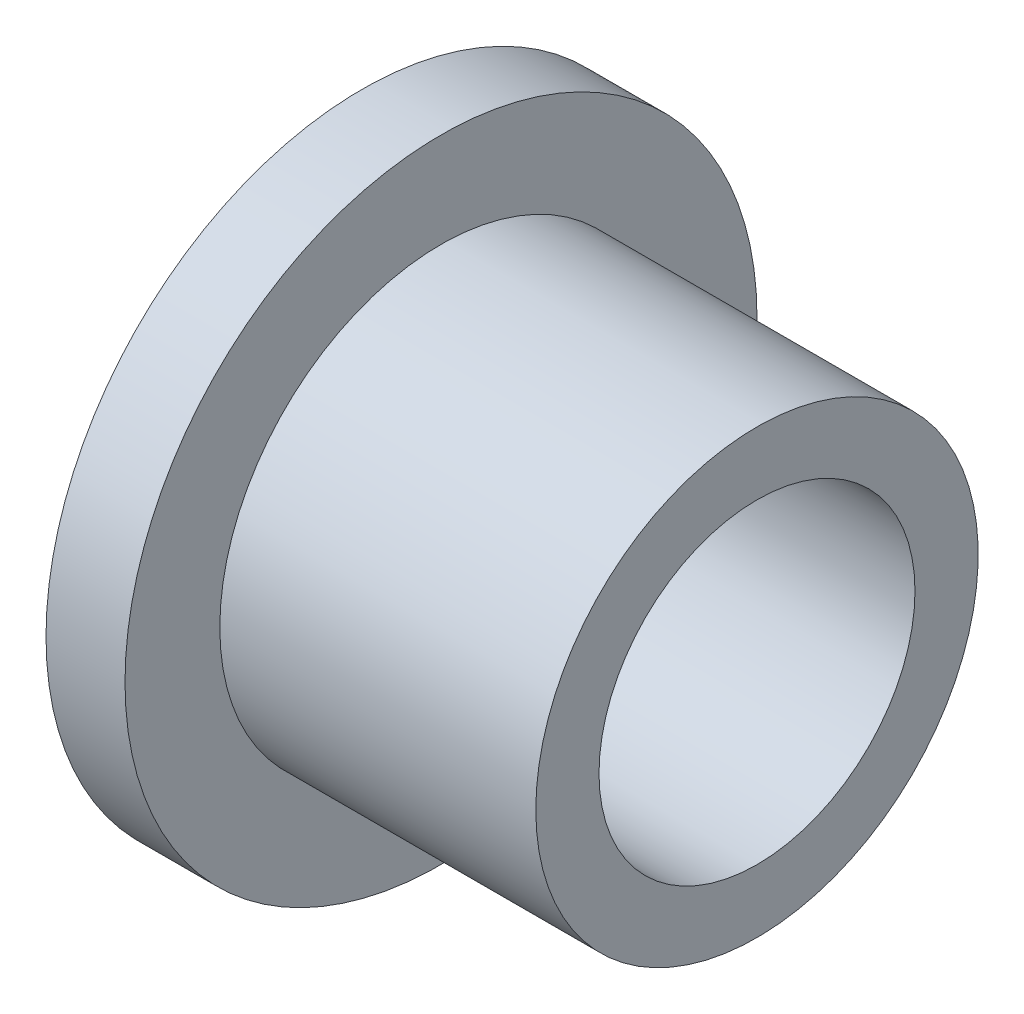
SolidWorks part; units mm, degrees
ref_plane "Front Plane" through (0, 0, 0) normal (0, 0, 1) x (1, 0, 0)
ref_plane "Top Plane" through (0, 0, 0) normal (0, 1, 0) x (1, 0, 0)
ref_plane "Right Plane" through (0, 0, 0) normal (1, 0, 0) x (0, 0, -1)
other "Configuration Table"
sketch "Sketch1" plane through (0, 0, 0) normal (0, 1, 0) x (1, 0, 0)
  line L0 (0, 0) -> (0, 10)
  line L1 (0, 10) -> (5, 10)
  line L2 (5, 10) -> (5, 4)
  line L3 (0, 0) -> (25, 0)
  line L4 (0, -10) -> (31.0824, -10) construction
  line L5 (5, 4) -> (25, 4)
  line L6 (25, 4) -> (25, 0)
  dimension "D1" = 10
  dimension "D2" = 14
  dimension "D3" = 20
  dimension "D4" = 5
  dimension "D5" = 25
revolve "Revolve1" add sketch "Sketch1" angle 360 about L4
